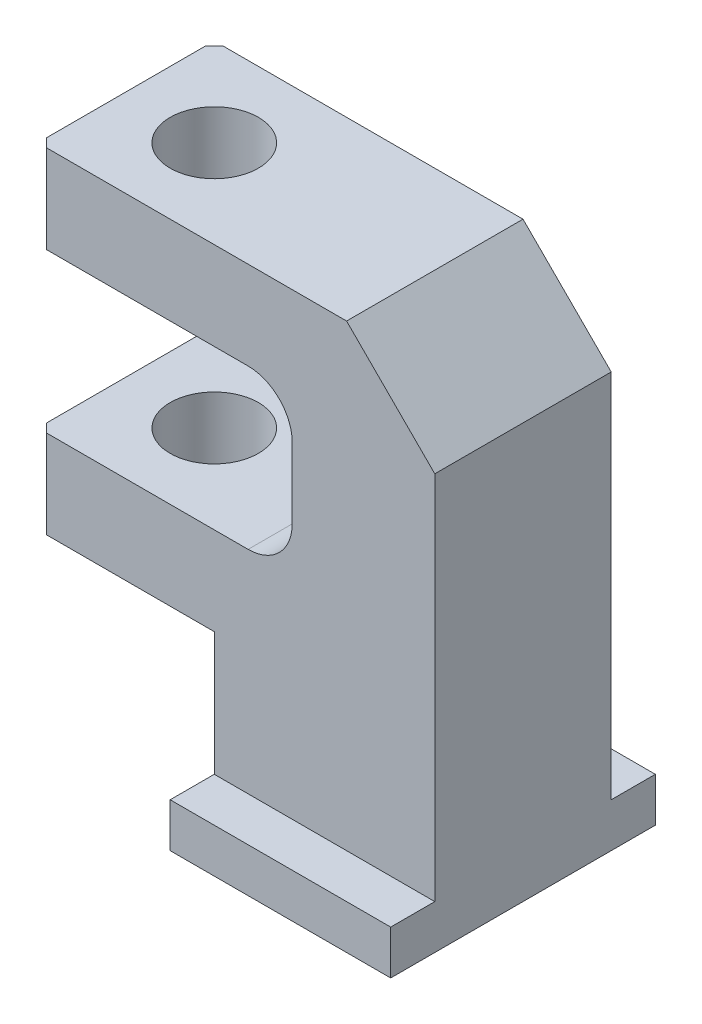
from build123d import *

# Parameters (mm, degrees)
SKETCH_1_W                  = 30
SKETCH_1_H                  = 57
EXTRUDE_1_DEPTH             = 25
SKETCH_2_W                  = 5
SKETCH_2_H                  = 52
CUT_EXTRUDE_1_DEPTH         = 65.02343321
SKETCH_3_W                  = 5
SKETCH_3_H                  = 52
CUT_EXTRUDE_2_DEPTH         = 65.02343321
SKETCH_4_W                  = 20
SKETCH_4_H                  = 38
EXTRUDE_2_DEPTH             = 20
SKETCH_5_W                  = 28.836169251
SKETCH_5_H                  = 18
CUT_EXTRUDE_3_DEPTH         = 69.190018281
HOLE_WIZARD_10_0_10_1_D     = 10
HOLE_WIZARD_10_0_10_1_DEPTH = 10
HOLE_WIZARD_10_0_10_2_D     = 10
HOLE_WIZARD_10_0_10_2_DEPTH = 38
HOLE_WIZARD_5_0_5_1_D       = 5
HOLE_WIZARD_5_0_5_1_DEPTH   = 17
HOLE_WIZARD_5_0_5_1_TIP     = 1.502151548
CHAMFER_1_SIZE              = 1
CHAMFER_2_SIZE              = 10
FILLET_1_R                  = 5


with BuildPart() as part:
    # 草图1 → 凸台-拉伸1 (new body)
    with BuildSketch(Plane(origin=(17.145402657, 0, 0), x_dir=(0, 0, -1), z_dir=(1, 0, 0))):
        with Locations((0, 28.5)):
            Rectangle(SKETCH_1_W, SKETCH_1_H)
    extrude(amount=-EXTRUDE_1_DEPTH)

    # 草图2 → 切除-拉伸1 (cut, through all)
    with BuildSketch(Plane(origin=(17.145402657, 0, 0), x_dir=(0, 0, -1), z_dir=(1, 0, 0))):
        with Locations((-12.5, 31)):
            Rectangle(SKETCH_2_W, SKETCH_2_H)
    extrude(amount=-CUT_EXTRUDE_1_DEPTH, mode=Mode.SUBTRACT)

    # 草图3 → 切除-拉伸2 (cut, through all)
    with BuildSketch(Plane(origin=(17.145402657, 0, 0), x_dir=(0, 0, -1), z_dir=(1, 0, 0))):
        with Locations((12.5, 31)):
            Rectangle(SKETCH_3_W, SKETCH_3_H)
    extrude(amount=-CUT_EXTRUDE_2_DEPTH, mode=Mode.SUBTRACT)

    # 草图4 → 凸台-拉伸2 (add)
    with BuildSketch(Plane.ZY.offset(7.854597343)):
        with Locations((0, 38)):
            Rectangle(SKETCH_4_W, SKETCH_4_H)
    extrude(amount=EXTRUDE_2_DEPTH)

    # 草图5 → 切除-拉伸3 (cut, through all)
    with BuildSketch(Plane.XY.offset(10)):
        with Locations((-13.436512718, 38)):
            Rectangle(SKETCH_5_W, SKETCH_5_H)
    extrude(amount=-CUT_EXTRUDE_3_DEPTH, mode=Mode.SUBTRACT)

    # Ø10.0 (10) 直径孔1
    with Locations(Plane(origin=(0, 47, 0), x_dir=(-1, 0, 0), z_dir=(0, -1, 0))):
        with Locations((17.854597343, 0)):
            Hole(HOLE_WIZARD_10_0_10_1_D / 2, depth=HOLE_WIZARD_10_0_10_1_DEPTH)

    # Ø10.0 (10) 直径孔2
    with Locations(Plane(origin=(0, 19, 0), x_dir=(-1, 0, 0), z_dir=(0, -1, 0))):
        with Locations((17.854597343, 0)):
            Hole(HOLE_WIZARD_10_0_10_2_D / 2, depth=HOLE_WIZARD_10_0_10_2_DEPTH)

    # Ø5.0 (5) 直径孔1
    with Locations(Plane(origin=(0, 0, 0), x_dir=(-1, 0, 0), z_dir=(0, -1, 0))):
        with Locations((2.854597343, 0), (-12.145402657, 0)):
            Hole(HOLE_WIZARD_5_0_5_1_D / 2, depth=HOLE_WIZARD_5_0_5_1_DEPTH)
            with Locations((0, 0, -(HOLE_WIZARD_5_0_5_1_DEPTH + HOLE_WIZARD_5_0_5_1_TIP / 2))):  # 118° drill point
                Cone(0, HOLE_WIZARD_5_0_5_1_D / 2, HOLE_WIZARD_5_0_5_1_TIP, mode=Mode.SUBTRACT)

    # 倒角1
    chamfer_1_edges = [part.edges().sort_by_distance(p)[0] for p in [
        (-27.854597343, 52, -10),
        (-27.854597343, 24, 10),
        (-27.854597343, 24, -10),
        (-27.854597343, 52, 10),
    ]]
    chamfer(chamfer_1_edges, length=CHAMFER_1_SIZE)

    # 倒角2
    chamfer_2_edges = [part.edges().sort_by_distance(p)[0] for p in [
        (17.145402657, 57, 0),
    ]]
    chamfer(chamfer_2_edges, length=CHAMFER_2_SIZE)

    # 圆角1
    fillet_1_edges = [part.edges().sort_by_distance(p)[0] for p in [
        (0.981571908, 47, 0),
        (0.981571908, 29, 0),
    ]]
    fillet(fillet_1_edges, radius=FILLET_1_R)


solid = part.part
